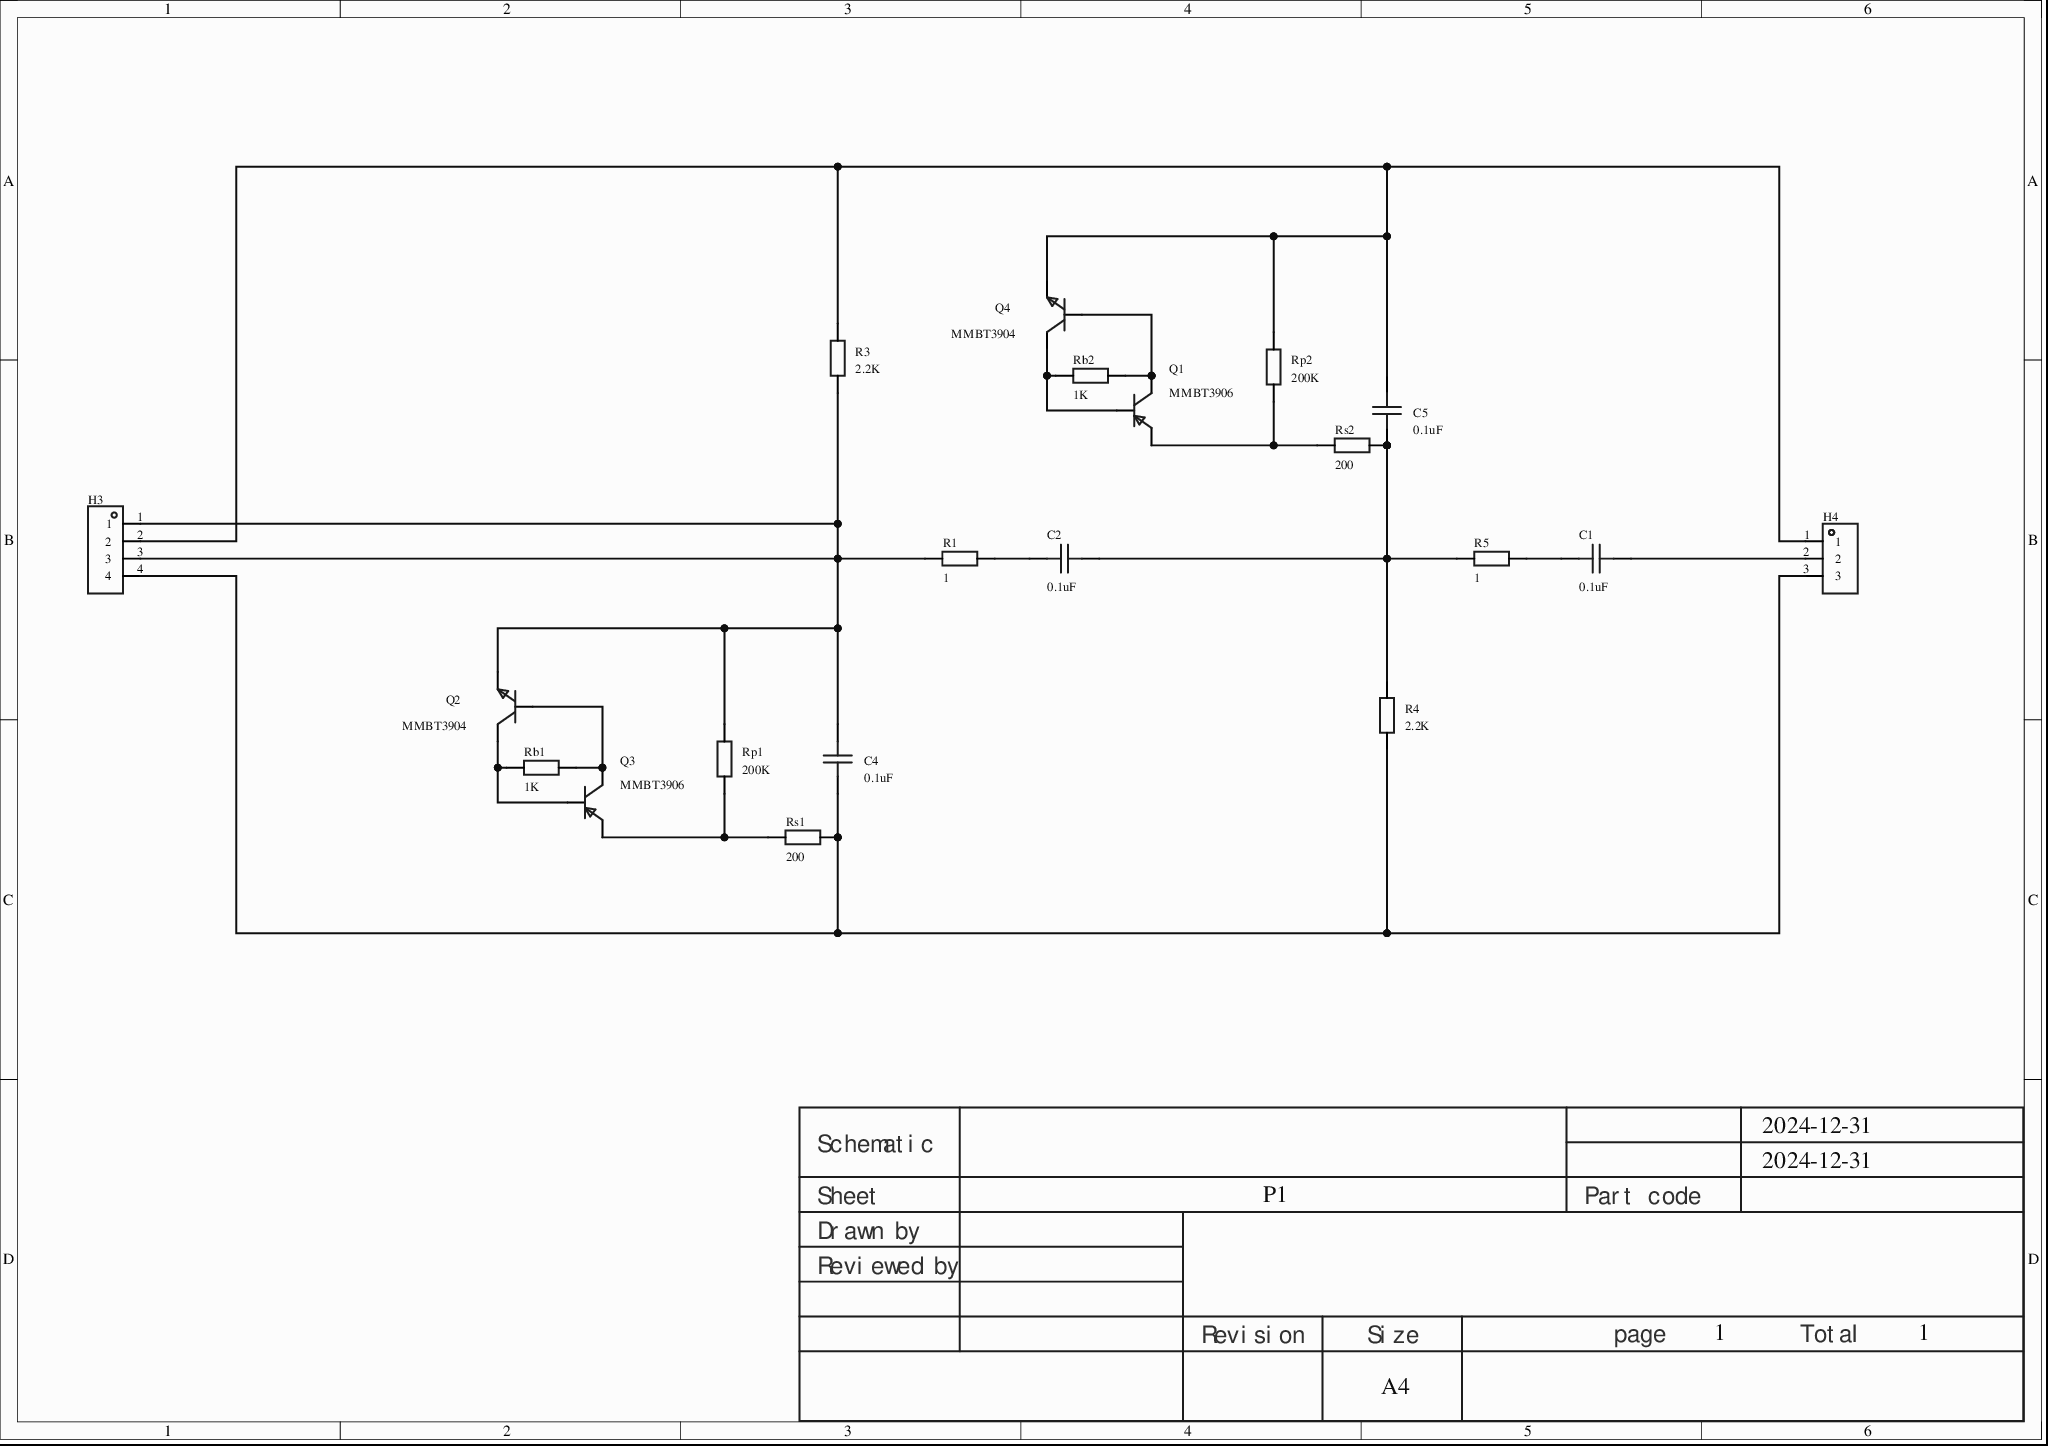
[diagram p0: MISC51661-3.schdoc]
# Altium project MISC51661-2.PrjPcb
1 sheet, 20 parts. Net scope: global (net labels, ports and power ports of the same name join across sheets).
Board file: MISC51661.pcbdoc

## Sheet MISC51661-3.schdoc
size 297 x 209 mm; Version: V1.0; @Project Name: MISC51661; @Page Count: 1; @Update Date: 2024-12-31; @Create Date: 2024-12-31; @Schematic Name: MISC51661; @Page No: 1; @Board Name: MISC51661; @Create Time: 12:48:38; @Update Time: 15:04:04

### Parts
C1  0.1uF  [C0402]
C2  0.1uF  [C0402]
C4  0.1uF  [C0402]
C5  0.1uF  [C0402]
H3  (no value)  [HDR-TH_4P-P2.54-V-M]
H4  (no value)  [HDR-TH_3P-P2.54-V-M]
Q1  MMBT3906  [SOT-23-3_L2.9-W1.3-P1.90-LS2.4-BR]
Q2  MMBT3904  [SOT-23-3_L2.9-W1.3-P1.90-LS2.4-BR]
Q3  MMBT3906  [SOT-23-3_L2.9-W1.3-P1.90-LS2.4-BR]
Q4  MMBT3904  [SOT-23-3_L2.9-W1.3-P1.90-LS2.4-BR]
R1  1  [R0402]
R3  2.2K  [R0402]
R4  2.2K  [R0402]
R5  1  [R0402]
Rb1  1K  [R0402]
Rb2  1K  [R0402]
Rp1  200K  [R0402]
Rp2  200K  [R0402]
Rs1  200  [R0402]
Rs2  200  [R0402]

### Nets
NetC1_1: C1.1 H4.2
NetC1_2: C1.2 R5.1
NetC2_1: C2.1 C5.1 R4.2 R5.2 Rs2.2
NetC2_2: C2.2 R1.1
NetC4_1: C4.1 H3.4 H4.3 R4.1 Rs1.2
NetC4_2: C4.2 H3.1 H3.3 Q2.2(E) R1.2 R3.1 Rp1.2
NetC5_2: C5.2 H3.2 H4.1 Q4.2(E) R3.2 Rp2.2
NetQ1_1: Q1.1(B) Q4.3(C) Rb2.2
NetQ1_2: Q1.2(E) Rp2.1 Rs2.1
NetQ1_3: Q1.3(C) Q4.1(B) Rb2.1
NetQ2_1: Q2.1(B) Q3.3(C) Rb1.1
NetQ2_3: Q2.3(C) Q3.1(B) Rb1.2
NetQ3_2: Q3.2(E) Rp1.1 Rs1.1

### Notes on the sheet
- 2024-12-31
- Schematic
- Sheet
- P1
- Part code
- Reviewed by
- Drawn by
- Revision
- Size
- A4
- page
- 1
- Total

### Library data of the parts
C1 C2 C4 C5 = CAP_0402: ConvertToPcb: yes; SymbolName: CapAcitance; ModelId: 36a51122f27c49738f86b3bfa98863e0; ModelName: C0402_L1.0-W0.5-H0.5; ModelTransform: 39.37,19.685,0,0,0,0,0,0,0; Value: 0.1uF; Device: CAP_0402; AddInBom: yes; Supplier Footprint: 0402; FootprintName: C0402
H3 = HDR-M_2.54_1x4P: Symbol: PZ254V-11-04P; ConvertToPcb: yes; ModelId: 112f4d05e8d64e99ab9a333894bea4f9; ModelName: HDR-TH_4P-P2.54-M-LI-1X4P; ModelTransform: 399.999,104.7242,0,0,0,0,0,0,-118.11; Device: HDR-M_2.54_1x4P; AddInBom: yes; SupplierPart: C492403; Supplier Footprint: 插件; FootprintName: HDR-TH_4P-P2.54-V-M
H4 = HDR-M_2.54_1x3P: Symbol: PZ254V-11-03P_C2937625; ConvertToPcb: yes; ModelId: bb473b6d38ff42a99216a4fcdbdcc4cb; ModelName: HDR-TH_3P-P2.54-M-LI-1X3P; ModelTransform: 299.9994,100,0,0,0,0,0,0,-118.11; Device: HDR-M_2.54_1x3P; AddInBom: yes; SupplierPart: C2937625; Supplier Footprint: 插件; FootprintName: HDR-TH_3P-P2.54-V-M
Q1 Q3 = MMBT3906-13-01-F: Transistor type: -; collector current (Ic): -; collector-emitter breakdown voltage (Vceo): -; power (Pd): -;; Manufacturer: DIODES(美台); AddInBom: yes; ModelId: c62791f0466c4ae2a892c056b845b0ca; ModelName: SOT-23-3P_L2.9-W1.3-H1.0-LS2.4-P0.95; ModelTransform: 98.425,114.173,0,180,0,0,0.0005,-0.0005,0; Symbol: MMBT3906-13-01-F; Manufacturer Part: MMBT3906; Device: MMBT3906-13-01-F; LCSC Part Name: MMBT3906-13-01-F; SupplierPart: C526675; Supplier Footprint: SOT-23-3; JLCPCB Part Class: Extended; Supplier: LCSC; ConvertToPcb: yes; FootprintName: SOT-23-3_L2.9-W1.3-P1.90-LS2.4-BR; Transistor Type: -; Collector Current (Ic): -; Collector-Emitter Breakdown Voltage (Vceo): -; Power Dissipation (Pd): -; Transition Frequency (fT): -; Collector Cut-Off Current (Icbo): -; Collector-Emitter Saturation Voltage (VCE(sat)@Ic,Ib): -
Q2 Q4 = MMBT3904(RANGE:100-300): Transistor type: NPN; collector current (Ic): 200mA; collector-emitter breakdown voltage (Vceo): 40V; power (Pd): 200mW; DC current gain (hFE@Ic,Vce): 100@10mA,1V;; Manufacturer: CJ(江苏长电/长晶); AddInBom: yes; ModelId: c62791f0466c4ae2a892c056b845b0ca; ModelName: SOT-23-3P_L2.9-W1.3-H1.0-LS2.4-P0.95; ModelTransform: 98.425,114.173,0,180,0,0,0.0005,-0.0005,0; Transition Frequency (fT): 300MHz; Collector Cut-Off Current (Icbo): 100nA; Collector-Emitter Saturation Voltage (VCE(sat)@Ic,Ib): 300mV@50mA,5mA; Symbol: MMBT3904; Manufacturer Part: MMBT3904; Device: MMBT3904(RANGE:100-300); LCSC Part Name: NPN 电流:200mA 耐压:40V hfe=100~300; SupplierPart: C20526; Supplier Footprint: SOT-23; Datasheet: https://atta.szlcsc.com/upload/public/pdf/source/20220704/70F575FB75061E03F919270A6BB8BA7F.pdf; Supplier: LCSC; ConvertToPcb: yes; FootprintName: SOT-23-3_L2.9-W1.3-P1.90-LS2.4-BR; Transistor Type: NPN; Collector Current (Ic): 200mA; Collector-Emitter Breakdown Voltage (Vceo): 40V; Power Dissipation (Pd): 200mW; DC Current Gain (hFE@Ic,Vce): 100@10mA,1V; Operating Temperature: -
R1 R3-R5 Rb1 Rb2 Rp1 Rp2 Rs1 Rs2 = Res_0402: Symbol: Resistor; ConvertToPcb: yes; ModelId: 671aefced39d4c318694bba8bd8efd39; ModelName: R0402_L1.0-W0.5-H0.5; ModelTransform: 39.37,19.685,0,0,0,0,0,0.0005,0; Device: Res_0402; AddInBom: yes; Supplier Footprint: 0402; FootprintName: R0402
  R1 R5: Value: 1
  R3 R4: Value: 2.2K
  Rb1 Rb2: Value: 1K
  Rp1 Rp2: Value: 200K
  Rs1 Rs2: Value: 200